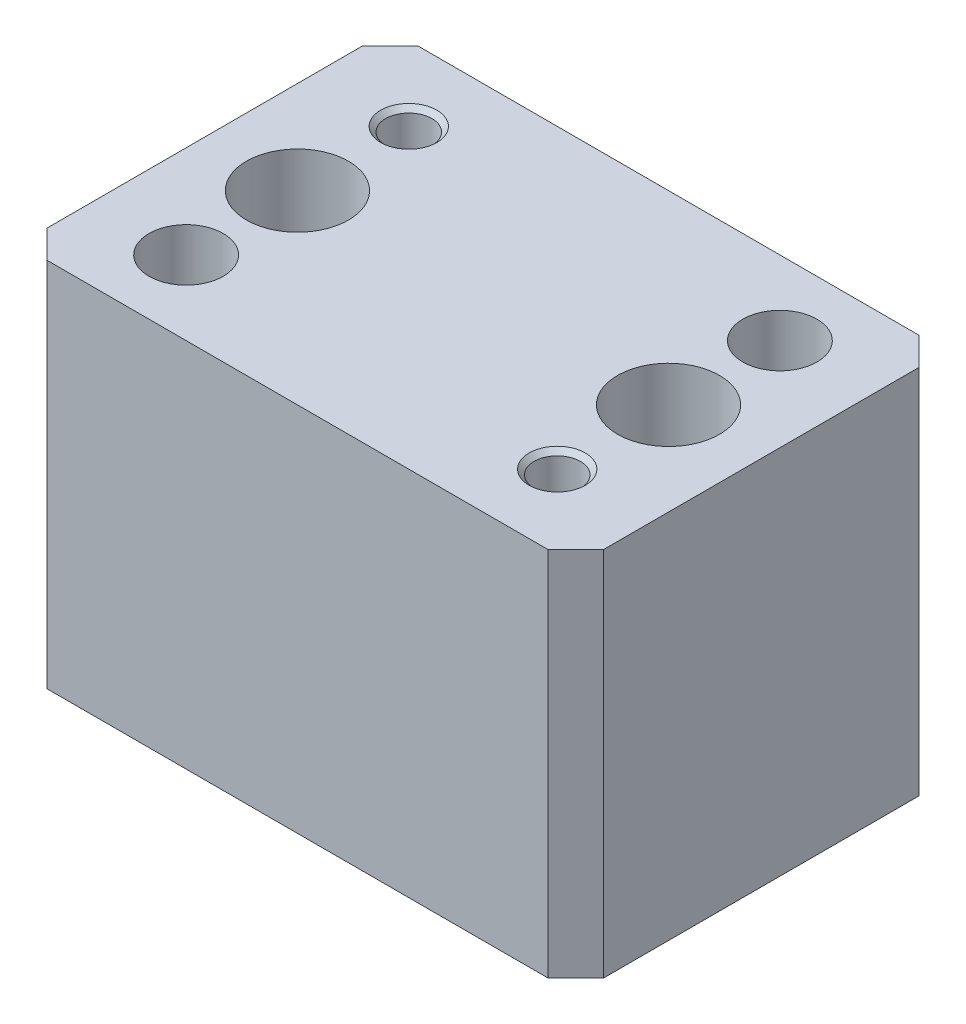
from build123d import *

# Parameters (mm, degrees)
SKETCH1_W                   = 60
SKETCH1_H                   = 40
BOSS_EXTRUDE1_DEPTH         = 40
CHAMFER1_SIZE               = 3
M6_TAPPED_HOLE1_D           = 5
M6_TAPPED_HOLE1_DEPTH       = 10.497848452
M6_TAPPED_HOLE1_CSINK_D     = 6.05
M6_TAPPED_HOLE1_CSINK_ANGLE = 90
M6_TAPPED_HOLE1_TIP         = 1.502151548
HOLE1_D                     = 6.6
HOLE1_CBORE_D               = 11
HOLE1_CBORE_DEPTH           = 27
HOLE2_D                     = 8
HOLE2_DEPTH                 = 9
HOLE3_D                     = 8
HOLE3_DEPTH                 = 8.5


with BuildPart() as part:
    # Sketch1 → Boss-Extrude1 (new body)
    with BuildSketch(Plane.XY):
        with Locations((-2.229013427, 0.789473684)):
            Rectangle(SKETCH1_W, SKETCH1_H)
    extrude(amount=BOSS_EXTRUDE1_DEPTH)

    # Chamfer1
    chamfer1_edges = [part.edges().sort_by_distance(p)[0] for p in [
        (27.770986573, 0.789473684, 40),
        (-32.229013427, 0.789473684, 40),
        (27.770986573, 0.789473684, 0),
        (-32.229013427, 0.789473684, 0),
    ]]
    chamfer(chamfer1_edges, length=CHAMFER1_SIZE)

    # M6 Tapped Hole1
    with Locations(Plane(origin=(0, 20.789473684, 0), x_dir=(1, 0, 0), z_dir=(0, 1, 0))):
        with Locations((-22.229013427, -8), (17.770986573, -32)):
            CounterSinkHole(M6_TAPPED_HOLE1_D / 2, M6_TAPPED_HOLE1_CSINK_D / 2, depth=M6_TAPPED_HOLE1_DEPTH, counter_sink_angle=M6_TAPPED_HOLE1_CSINK_ANGLE)
            with Locations((0, 0, -(M6_TAPPED_HOLE1_DEPTH + M6_TAPPED_HOLE1_TIP / 2))):  # 118° drill point
                Cone(0, M6_TAPPED_HOLE1_D / 2, M6_TAPPED_HOLE1_TIP, mode=Mode.SUBTRACT)

    # Hole1 (through all)
    with Locations(Plane(origin=(0, 20.789473684, 0), x_dir=(1, 0, 0), z_dir=(0, 1, 0))):
        with Locations((-22.229013427, -20), (17.770986573, -20)):
            CounterBoreHole(HOLE1_D / 2, HOLE1_CBORE_D / 2, HOLE1_CBORE_DEPTH)

    # Hole2
    with Locations(Plane(origin=(0, 20.789473684, 0), x_dir=(1, 0, 0), z_dir=(0, 1, 0))):
        with Locations((17.770986573, -8), (-22.229013427, -32)):
            Hole(HOLE2_D / 2, depth=HOLE2_DEPTH)

    # Hole3
    with Locations(Plane(origin=(0, -19.210526316, 0), x_dir=(-1, 0, 0), z_dir=(0, -1, 0))):
        with Locations((2.229013427, -34), (2.229013427, -6)):
            Hole(HOLE3_D / 2, depth=HOLE3_DEPTH)


solid = part.part
